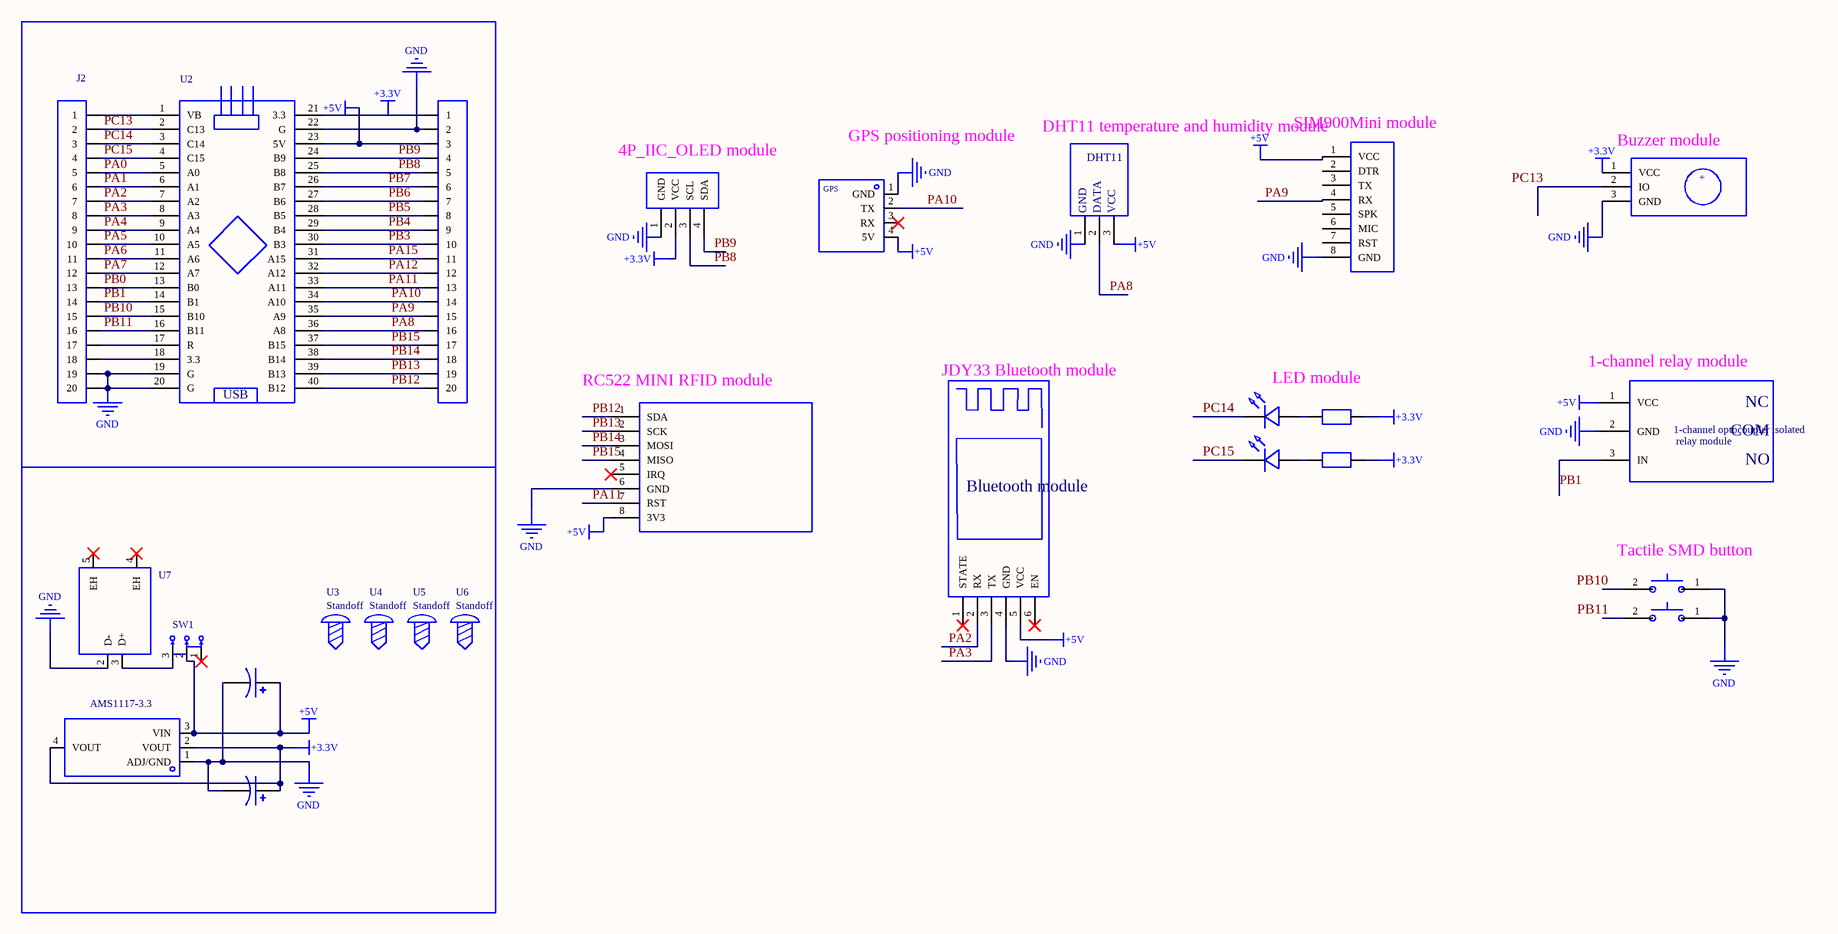
[diagram p0: MISC49937-3.schdoc]
# Altium project MISC49937-2.PrjPcb
1 sheet, 26 parts. Net scope: global (net labels, ports and power ports of the same name join across sheets).
Board file: MISC49937.pcbdoc

## Sheet MISC49937-3.schdoc
size 420 x 298 mm; Version: V1.0; @Project Name: MISC49937; @Page Count: 1; @Update Date: 2026-01-31; @Create Date: 2026-01-31; @Schematic Name: MISC49937; @Page No: 1

### Parts
1  FYS#DHT11 COPY  [FYS#DHT11_X COPY]  (value not drawn)
C1  1u  [CAP-D3.0×F1.5]  (value not drawn)
C2  1u  [CAP-D3.0×F1.5]  (value not drawn)
J1  HDR-M-2.54_1x20  [HDR-M-2.54_1X20]  (value not drawn)
J2  HDR-M-2.54_1x20  [HDR-M-2.54_1X20]  (value not drawn)
LED1  LED-TH-3mm_R  [LED-TH_BD3.0_RED]  (value not drawn)
LED2  LED-TH-3mm_R  [LED-TH_BD3.0_RED]  (value not drawn)
R1  1k  [R_AXIAL-0.3]  (value not drawn)
R2  1k  [R_AXIAL-0.3]  (value not drawn)
SW1  SS12D00G3  [SW-TH_SS-12D01-GX]  (value not drawn)
SW2  1TS002B-2300-5001  [SW-SMD_L6.0-W3.5-LS8.0]  (value not drawn)
SW3  1TS002B-2300-5001  [SW-SMD_L6.0-W3.5-LS8.0]  (value not drawn)
U1  AMS1117-3.3  [SOT-223_L6.5-W3.5-P2.30-LS7.0-BR]
U2  (no value)  [FYS_STM32F103C最小系统]
U3  Standoff  [M3铜柱]
U4  Standoff  [M3铜柱]
U5  Standoff  [M3铜柱]
U6  Standoff  [M3铜柱]
U7  TYPE-C 2P 90 2J 108  [usb-a-th_type-c-2p-90-2j-108]  (value not drawn)
U8  FYS#0.96 OLED IIC_4PIN COPY COPY COPY  [FYS_OLED_IIC]  (value not drawn)
U9  FYS#GPS-6M_no mounting hole  [FYS#GPS模块_不带槽]  (value not drawn)
U10  FYS#SIM900AMINI  [FYS#SIM900AMINI]  (value not drawn)
U11  FYS#RC522 MINI RFID module COPY COPY  [FYS#RC522 MINI RFID模块 COPY_1]  (value not drawn)
U12  FYS#HC series Bluetooth module COPY  [FYS#HC-05蓝牙模块 COPY]  (value not drawn)
U13  FYS#BEEP buzzer module COPY  [FYS#BEEP蜂鸣器模块 COPY]  (value not drawn)
U14  FYS#1-channel 5V optocoupler isolated relay module COPY  [FYS#1路5V光偶隔离继电器模块 COPY]  (value not drawn)

### Nets
+3.3V: C2.1 J1.1 R1.2 R2.2 U1.2(VOUT) U1.4(VOUT) U2.21(3.3) U8.2(VCC) U13.1(VCC)
+5V: 1.3(VCC) C1.1 J1.3 SW1.2 U1.3(VIN) U2.23(5V) U9.4(5V) U10.1(VCC) U11.8(3V3) U12.5(VCC) U14.1(VCC)
GND: 1.1(GND) C1.2 C2.2 J1.2 J2.19 J2.20 SW2.1(A) SW3.1(A) U1.1(ADJ/GND) U2.19(G) U2.20(G) U2.22(G) U7.2(D-) U8.1(GND) U9.1(GND) U10.8(GND) U11.6(GND) U12.4(GND) U13.3(GND) U14.2(GND)
PA0: J2.5 U2.5(A0)
PA1: J2.6 U2.6(A1)
PA2: J2.7 U2.7(A2) U12.2(RX)
PA3: J2.8 U2.8(A3) U12.3(TX)
PA4: J2.9 U2.9(A4)
PA5: J2.10 U2.10(A5)
PA6: J2.11 U2.11(A6)
PA7: J2.12 U2.12(A7)
PA8: 1.2(DATA) J1.16 U2.36(A8)
PA9: J1.15 U2.35(A9) U10.4(RX)
PA10: J1.14 U2.34(A10) U9.2(TX)
PA11: J1.13 U2.33(A11) U11.7(RST)
PA12: J1.12 U2.32(A12)
PA15: J1.11 U2.31(A15)
PB0: J2.13 U2.13(B0)
PB1: J2.14 U2.14(B1) U14.3(IN)
PB3: J1.10 U2.30(B3)
PB4: J1.9 U2.29(B4)
PB5: J1.8 U2.28(B5)
PB6: J1.7 U2.27(B6)
PB7: J1.6 U2.26(B7)
PB8: J1.5 U2.25(B8) U8.3(SCL)
PB9: J1.4 U2.24(B9) U8.4(SDA)
PB10: J2.15 SW2.2(B) U2.15(B10)
PB11: J2.16 SW3.2(B) U2.16(B11)
PB12: J1.20 U2.40(B12) U11.1(SDA)
PB13: J1.19 U2.39(B13) U11.2(SCK)
PB14: J1.18 U2.38(B14) U11.3(MOSI)
PB15: J1.17 U2.37(B15) U11.4(MISO)
PC13: J2.2 U2.2(C13) U13.2(IO)
PC14: J2.3 LED1.2 U2.3(C14)
PC15: J2.4 LED2.2 U2.4(C15)
NetJ2_1: J2.1 U2.1(VB)
NetJ2_17: J2.17 U2.17(R)
NetJ2_18: J2.18 U2.18(3.3)
NetLED1_1: LED1.1 R1.1
NetLED2_1: LED2.1 R2.1
NetSW1_3: SW1.3 U7.3(D+)

Not connected (* = marked no-connect by the designer): SW1 1*; U7 4(EH)* 5(EH)*; U9 3(RX)*; U10 2(DTR) 3(TX) 5(SPK) 6(MIC) 7(RST); U11 5(IRQ)*; U12 1(STATE)* 6(EN)*

### Notes on the sheet
- (near U10) DHT11 temperature and humidity module
- (near U10) SIM900Mini module
- (near U8) 4P_IIC_OLED module
- (near U9) GPS positioning module
- (near U13) Buzzer module
- (near U11) RC522 MINI RFID module
- JDY33 Bluetooth module
- LED module
- (near U14) 1-channel relay module
- (near SW2) Tactile SMD button
- 2026-01-31
- Schematic
- Sheet
- P1
- Material code
- Checked
- Drawn
- Revision
- Size
- A3
- page
- 1
- Total

### Library data of the parts
1 = FYS#DHT11 COPY: Add into BOM: yes; Symbol: FYS#DHT11 COPY; Device: FYS#DHT11 COPY; Convert to PCB: yes; Origin Footprint: FYS#DHT11_X COPY; FootprintName: FYS#DHT11_X COPY
C1 C2 = 1u: Add into BOM: yes; Symbol: 1u; Device: 1u; Convert to PCB: yes; Origin Footprint: CAP-D3.0×F1.5; FootprintName: CAP-D3.0×F1.5
J1 = HDR-M-2.54_1x20: Add into BOM: yes; ModelId: 3a23733f0ee3481e9756e4311e8a6823; Symbol: HDR-M-2.54_1x20; Device: HDR-M-2.54_1x20; Convert to PCB: yes; Origin Footprint: HDR-M-2.54_1X20; Supplier Part: C50981; Supplier: LCSC; FootprintName: HDR-M-2.54_1X20; ModelName: HDR-M-2.54_1x20
J2 = HDR-M-2.54_1x20_1: Add into BOM: yes; ModelId: 3a23733f0ee3481e9756e4311e8a6823; Symbol: HDR-M-2.54_1x20_1; Device: HDR-M-2.54_1x20_1; Convert to PCB: yes; Origin Footprint: HDR-M-2.54_1X20; Supplier Part: C50981; Supplier: LCSC; FootprintName: HDR-M-2.54_1X20; ModelName: HDR-M-2.54_1x20
LED1 LED2 = LED-TH-3mm_R: Manufacturer: EVERLIGHT(台湾亿光); Manufacturer Part: 204-10SDRD/S530-A3-L; Add into BOM: yes; ModelId: f7fa6dc8d0ed4ec283a3b0ca58a3d13c; Symbol: LED-TH-3mm_R; Device: LED-TH-3mm_R; Convert to PCB: yes; Origin Footprint: LED-TH_BD3.0_RED; Supplier Part: C84774; Supplier: LCSC; FootprintName: LED-TH_BD3.0_RED; ModelName: LED-TH_BD3.0_Red
R1 R2 = 1k: Add into BOM: yes; ModelId: 3f997efe3b344f2d8e0a2d7f24a0763d; Symbol: 1k; Device: 1k; Convert to PCB: yes; Origin Footprint: R_AXIAL-0.3; FootprintName: R_AXIAL-0.3; ModelName: R_AXIAL-0.3
SW1 = SS12D00G3: Manufacturer: null; Add into BOM: yes; ModelId: 46ec4e06866345239622c383c14b792d; Symbol: SS12D00G3; Device: SS12D00G3; Convert to PCB: yes; Origin Footprint: SW-TH_SS-12D01-GX; Supplier: LCSC; Supplier Part: C9900018735; Manufacturer Part: SS12D00G3; JLCPCB Part Class: Extended Part; FootprintName: SW-TH_SS-12D01-GX; ModelName: SW-TH_SS-12D01-GX
SW2 SW3 = 1TS002B-2300-5001: Manufacturer: HYP(鸿源精密); Manufacturer Part: 1TS002B-2300-5001-CT; Add into BOM: yes; Convert to PCB: yes; Origin Footprint: SW-SMD_L6.0-W3.5-LS8.0; Supplier: LCSC; Supplier Part: C319332; JLCPCB Part Class: Extended Part; Symbol: 1TS002B-2300-5001; Device: 1TS002B-2300-5001; FootprintName: SW-SMD_L6.0-W3.5-LS8.0
U1 = AMS1117-3.3: Manufacturer: PUOLOP(迪浦); Add into BOM: yes; Symbol: AMS1117-3.3; Device: AMS1117-3.3; Convert to PCB: yes; Origin Footprint: SOT-223_L6.5-W3.5-P2.30-LS7.0-BR; Supplier: LCSC; Supplier Part: C351785; Manufacturer Part: AMS1117-3.3; JLCPCB Part Class: Extended Part; FootprintName: SOT-223_L6.5-W3.5-P2.30-LS7.0-BR
U2 = FYS_STM32F103C最小系统: Symbol: FYS_STM32F103C minimum system; AddInBom: yes; Device: FYS_STM32F103C minimum system; Supplier: FYS; ConvertToPcb: yes; FootprintName: FYS_STM32F103C minimum system
U3-U6 = 铜柱: Add into BOM: yes; Origin Footprint: M3 standoff; Symbol: Standoff; Device: Standoff; Convert to PCB: yes; FootprintName: M3 standoff
U7 = TYPE-C 2P 90 2J 108: 连接器类型:Type-C;公母:母;安装方式:弯插;触点数量:2P;端口数量:1;额定电流 - 电源:3A;触头材质:铜;触头镀层:金;工作温度范围:-20℃~+85℃;; Manufacturer: SHOU HAN(首韩); 3D Model: bd78a49a637e45cdb15e881a0a048583; 3D Model Transform: 352.362,253.149,0,0,0,0,-0.001,-42.126,-62.992; Gender: Female; Number of Ports: 1; Current Rating - Power (Max): 3A; Rated Voltage (Max): 5V; Connect-Disconnect Life: 5 thousand cycles; Core Colour: Black; AddInBom: yes; Symbol: type-c 2p 90 2j 108; Device: TYPE-C 2P 90 2J 108; LCSC Part Name: Type-C 母 弯插; Supplier Part: C30167320; Manufacturer Part: TYPE-C 2P 90 2J 108; Supplier Footprint: 插件; JLCPCB Part Class: Extended library; Datasheet: https://atta.szlcsc.com/upload/public/pdf/source/20240719/36C790864DBB9824C105AFE70BC982EC.pdf; Supplier: LCSC; Connector Type: Type-C; Mounting Style: Right angle; Number of Contacts: 2P; Contact Material: Copper; Contact Plating: Gold; Operating Temperature Range: -20℃~+85℃; Length: 6.43mm; ConvertToPcb: yes; FootprintName: usb-a-th_type-c-2p-90-2j-108; ModelName: USB-A-TH_TYPE-C-2P-90-2J-108
U8 = FYS#0.96 OLED IIC_4PIN COPY COPY COPY: Add into BOM: yes; Symbol: FYS#0.96 OLED IIC_4PIN COPY COPY COPY; Device: FYS#0.96 OLED IIC_4PIN COPY COPY COPY; Convert to PCB: yes; Origin Footprint: FYS_OLED_IIC; FootprintName: FYS_OLED_IIC
U9 = FYS#GPS-6M_不带固定孔: Add into BOM: yes; Origin Footprint: FYS#GPS module_no slot; Symbol: FYS#GPS-6M_no mounting hole; Device: FYS#GPS-6M_no mounting hole; Convert to PCB: yes; FootprintName: FYS#GPS module_no slot
U10 = FYS#SIM900AMINI: Manufacturer: lengyuefeng; Add into BOM: yes; Symbol: FYS#SIM900AMINI; Device: FYS#SIM900AMINI; Convert to PCB: yes; Origin Footprint: FYS#SIM900AMINI; FootprintName: FYS#SIM900AMINI; Supplier: lengyuefeng
U11 = FYS#RC522 MINI RFID模块 COPY COPY_1: Symbol: FYS#RC522 MINI RFID module COPY COPY_1; Add into BOM: yes; Device: FYS#RC522 MINI RFID module COPY COPY_1; Convert to PCB: yes; Origin Footprint: FYS#RC522 MINI RFID module COPY; Supplier: Rysim; FootprintName: FYS#RC522 MINI RFID module COPY_1
U12 = FYS#HC系列蓝牙模块 COPY: Add into BOM: yes; Origin Footprint: FYS#HC-05 Bluetooth module COPY; Symbol: FYS#HC series Bluetooth module COPY; Device: FYS#HC series Bluetooth module COPY; Convert to PCB: yes; FootprintName: FYS#HC-05 Bluetooth module COPY
U13 = FYS#BEEP蜂鸣器模块 COPY: Add into BOM: yes; Symbol: FYS#BEEP buzzer module COPY; Device: FYS#BEEP buzzer module COPY; Convert to PCB: yes; Origin Footprint: FYS#BEEP buzzer module COPY; FootprintName: FYS#BEEP buzzer module COPY
U14 = FYS#1路5V光偶隔离继电器模块 COPY: Add into BOM: yes; Symbol: FYS#1-channel 5V optocoupler isolated relay module COPY; Device: FYS#1-channel 5V optocoupler isolated relay module COPY; Convert to PCB: yes; Origin Footprint: FYS#1-channel 5V optocoupler isolated relay module COPY; FootprintName: FYS#1-channel 5V optocoupler isolated relay module COPY